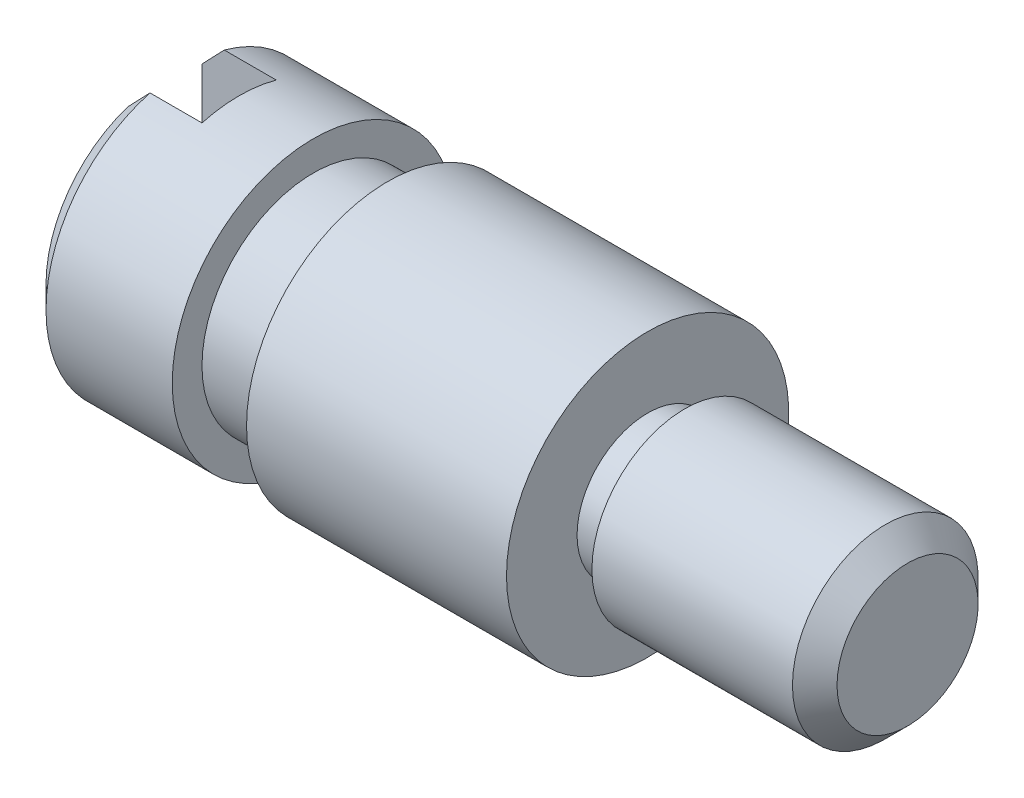
SolidWorks part; units mm, degrees
material "SUS 303"
ref_plane "Front Plane" through (0, 0, 0) normal (0, 0, 1) x (1, 0, 0)
ref_plane "Top Plane" through (0, 0, 0) normal (0, 1, 0) x (1, 0, 0)
ref_plane "Right Plane" through (0, 0, 0) normal (1, 0, 0) x (0, 0, -1)
sketch "Sketch1" plane through (0, 0, 0) normal (0, 1, 0) x (1, 0, 0)
  line L0 (0, 0) -> (-10, 0)
  line L1 (-10, 0) -> (-10, 1.6)
  line L2 (-9.7, 1.9) -> (-8, 1.9)
  line L3 (-8, 1.9) -> (-8, 1.5)
  line L4 (-8, 1.5) -> (-7, 1.5)
  line L5 (-7, 1.5) -> (-7, 1.9)
  line L6 (-7, 1.9) -> (-3.5, 1.9)
  line L7 (-3.5, 1.9) -> (-3.5, 0.95)
  line L8 (-3, 1.25) -> (-0.3, 1.25)
  line L9 (0, 0.95) -> (0, 0)
  line L10 (0, 0) -> (7.0515, 0) construction
  line L11 (-3, 1.25) -> (-3, 0.95)
  line L12 (-3, 0.95) -> (-3.5, 0.95)
  line L13 (-0.3, 1.25) -> (0, 0.95)
  line L14 (-10, 1.6) -> (-9.7, 1.9)
  point P4 (-10, 1.9)
  point P11 (0, 1.25)
  dimension "D1" = 3.8
  dimension "D2" = 3.8
  dimension "D3" = 3
  dimension "D4" = 2.5
  dimension "D5" = 10
  dimension "D6" = 2
  dimension "D7" = 1
  dimension "D8" = 3.5
  dimension "D9" = 0.5
  dimension "D10" = 0.3
revolve "Revolve1" add sketch "Sketch1" angle 360 about L10
cosmetic thread "Cosmetic Thread1"
sketch "Sketch2" plane through (-10, 0, 0) normal (-1, 0, 0) x (0, 0, 1)
  line L1 (-0.5, 3.3885) -> (0.5, 3.3885)
  line L2 (-0.5, 3.3885) -> (-0.5, -3.3885)
  line L3 (-0.5, -3.3885) -> (0.5, -3.3885)
  line L4 (0.5, 3.3885) -> (0.5, -3.3885)
  line L5 (-0.5, 3.3885) -> (0.5, -3.3885) construction
  line L6 (-0.5, -3.3885) -> (0.5, 3.3885) construction
  point P0 (0, 0)
  dimension "D1" = 1
extrude "Cut-Extrude1" cut sketch "Sketch2" against normal blind 1
